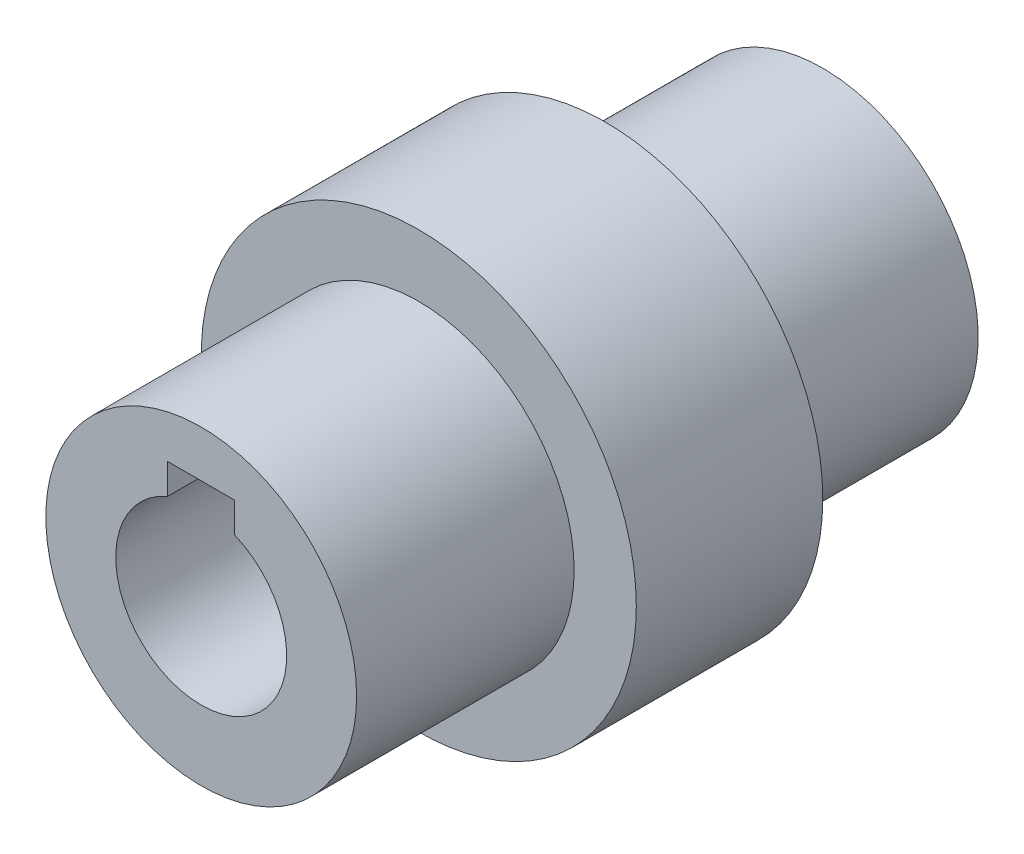
SolidWorks part; units mm, degrees
ref_plane "前视基准面" through (0, 0, 0) normal (0, 0, 1) x (1, 0, 0)
ref_plane "上视基准面" through (0, 0, 0) normal (0, 1, 0) x (1, 0, 0)
ref_plane "右视基准面" through (0, 0, 0) normal (1, 0, 0) x (0, 0, -1)
other "Configuration Table"
sketch "草图1" plane through (0, 0, 0) normal (0, 0, 1) x (1, 0, 0)
  circle A0 centre (0, 0) radius 35
  dimension "D1" = 70
extrude "凸台-拉伸1" add sketch "草图1" along normal mid plane 30 contours A0
sketch "草图2" plane through (0, 0, 15) normal (0, 0, 1) x (1, 0, 0)
  circle A0 centre (0, 0) radius 25
  dimension "D1" = 50
extrude "凸台-拉伸2" add sketch "草图2" along normal blind 35 contours A0
sketch "草图3" plane through (0, 0, -15) normal (0, 0, -1) x (-1, 0, 0)
  circle A0 centre (0, 0) radius 25 construction
  circle A1 centre (0, 0) radius 25
extrude "凸台-拉伸3" add sketch "草图3" along normal blind 35 contours A1
sketch "草图4" plane through (0, 0, 50) normal (0, 0, 1) x (1, 0, 0)
  line L1 (-5.385, 17.5) -> (5.385, 17.5)
  line L2 (-5.385, 17.5) -> (-5.385, 12.6517)
  line L4 (5.385, 17.5) -> (5.385, 12.6517)
  arc A0 (-5.385, 12.6517) -> (5.385, 12.6517) centre (0, 0) ccw
  point P1 (0, 0)
  point P4 (0, 0)
  point P8 (0, 17.5)
  dimension "D1" = 27.5
  dimension "D2" = 10.77
  dimension "D3" = 17.5
extrude "切除-拉伸1" cut sketch "草图4" against normal mid plane 50 contours A0 L4 L1 L2
sketch "草图5" plane through (0, 0, -50) normal (0, 0, -1) x (-1, 0, 0)
  circle A0 centre (0, 0) radius 12.5
  dimension "D1" = 25
extrude "切除-拉伸2" cut sketch "草图5" against normal mid plane 50 contours A0
sketch "草图6" plane through (0, 0, -50) normal (0, 0, -1) x (-1, 0, 0)
  line L1 (-5, 15) -> (5, 15)
  line L2 (-5, 15) -> (-5, 11.4564)
  line L4 (5, 15) -> (5, 11.4564)
  circle A0 centre (0, 0) radius 12.5 construction
  arc A1 (5, 11.4564) -> (-5, 11.4564) centre (0, 0) ccw
  dimension "D1" = 10
  dimension "D2" = 15
  dimension "D3" = 5
extrude "切除-拉伸3" cut sketch "草图6" against normal mid plane 30 contours L4 A1 L2 L1
